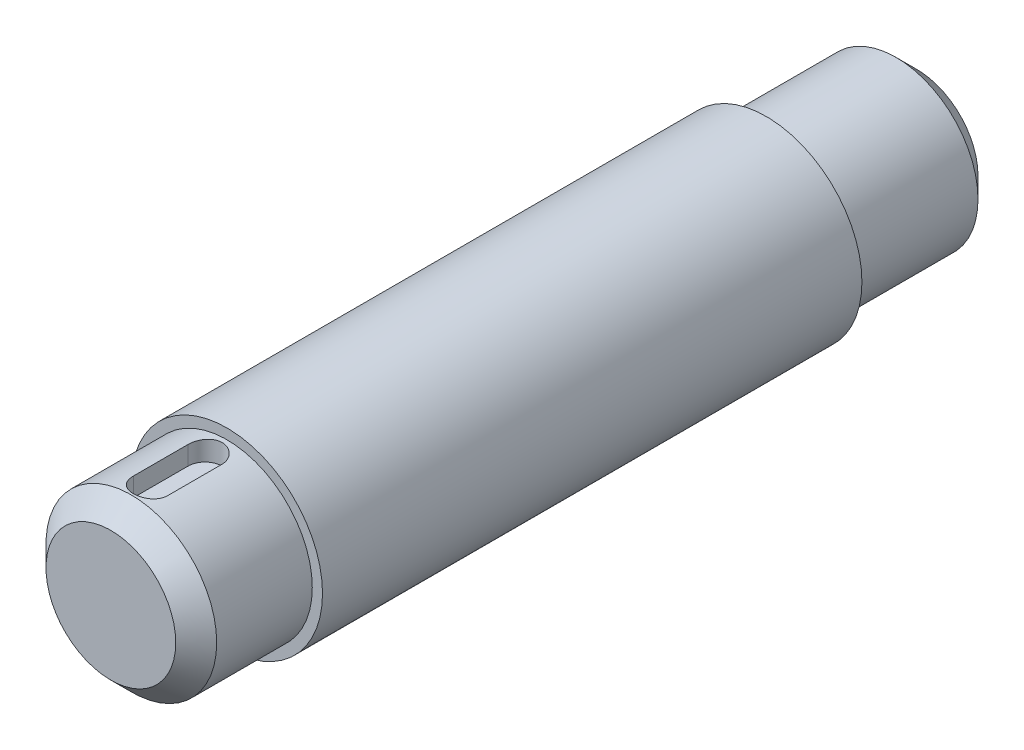
SolidWorks part; units mm, degrees
ref_plane "Front Plane" through (0, 0, 0) normal (0, 0, 1) x (1, 0, 0)
ref_plane "Top Plane" through (0, 0, 0) normal (0, 1, 0) x (1, 0, 0)
ref_plane "Right Plane" through (0, 0, 0) normal (1, 0, 0) x (0, 0, -1)
sketch "Sketch1" plane through (0, 0, 0) normal (0, 0, 1) x (1, 0, 0)
  circle A0 centre (0, 0) radius 12
extrude "Boss-Extrude1" add sketch "Sketch1" against normal blind 22
sketch "Sketch2" plane through (0, 0, 0) normal (0, 0, 1) x (1, 0, 0)
  circle A0 centre (0, 0) radius 14
  dimension "D1" = 28
extrude "Boss-Extrude2" add sketch "Sketch2" along normal blind 96
sketch "Sketch3" plane through (0, 0, 96) normal (0, 0, 1) x (1, 0, 0)
  circle A0 centre (0, 0) radius 12.5
  circle A1 centre (0, 0) radius 14 construction
  circle A2 centre (0, 0) radius 14
  dimension "D1" = 25
extrude "Cut-Extrude1" cut sketch "Sketch3" against normal blind 66
chamfer "Chamfer1" distance 3 angle 45 2 edges at (12.5, 0, 96) (12, 0, -22)
other "Move Face1" face at (12.5, 0, 30) parameters "D1"=49
ref_plane "Plane1" through (0, 12.5, 0) normal (0, 1, 0) x (1, 0, 0)
sketch "Sketch4" plane through (0, 12.5, 0) normal (0, 1, 0) x (1, 0, 0)
  line L0 (0, -90.2) -> (0, -82.2) construction
  line L2 (-2.5, -90.2) -> (-2.5, -82.2)
  line L3 (2.5, -90.2) -> (2.5, -82.2)
  line L4 (12.5, -93) -> (-12.5, -93) construction
  arc A0 (-2.5, -90.2) -> (2.5, -90.2) centre (0, -90.2) ccw
  arc A1 (2.5, -82.2) -> (-2.5, -82.2) centre (0, -82.2) ccw
  point P5 (0, -86.2)
  dimension "D1" = 5
  dimension "D2" = 8
  dimension "D3" = 6.8
extrude "Cut-Extrude2" cut sketch "Sketch4" against normal blind 3
